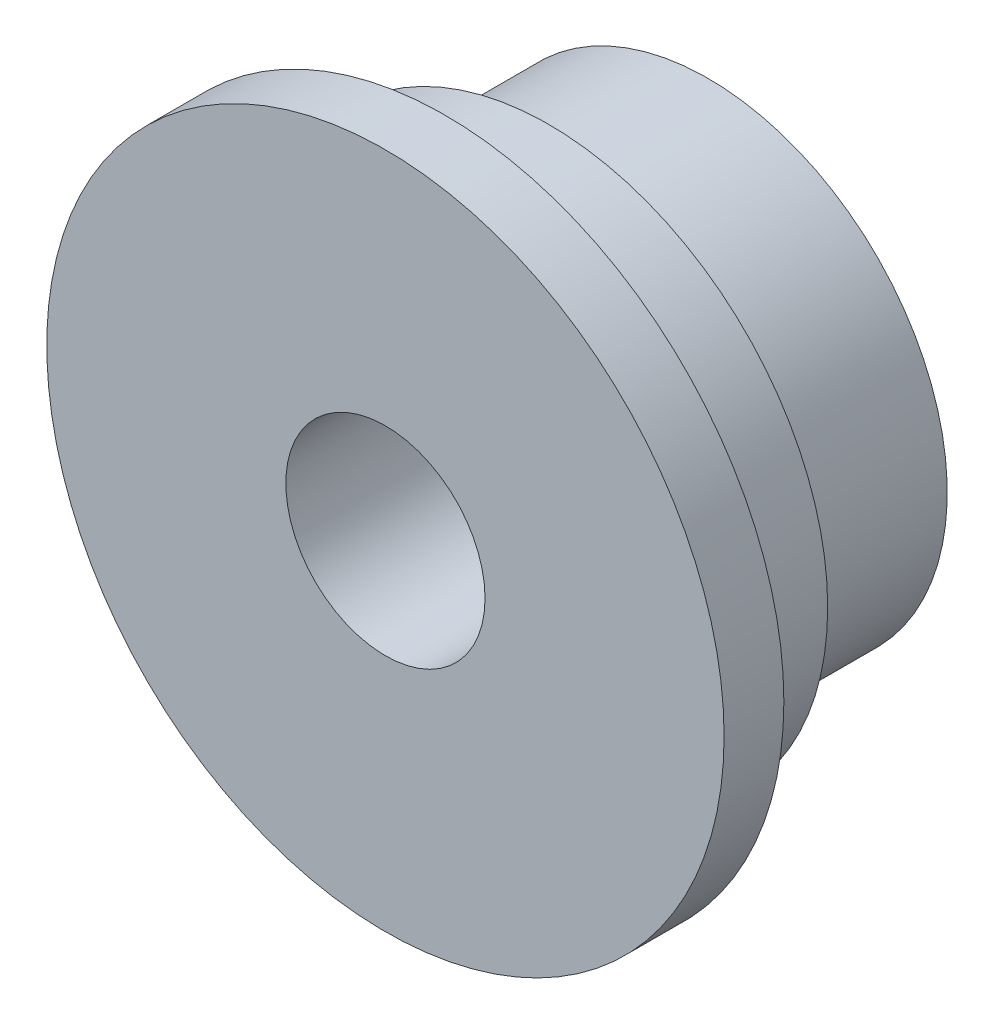
SolidWorks part; units mm, degrees
ref_plane "Front Plane" through (0, 0, 0) normal (0, 0, 1) x (1, 0, 0)
ref_plane "Top Plane" through (0, 0, 0) normal (0, 1, 0) x (1, 0, 0)
ref_plane "Right Plane" through (0, 0, 0) normal (1, 0, 0) x (0, 0, -1)
other "Configuration Table"
sketch "Sketch1" plane through (0, 0, 0) normal (0, 0, 1) x (1, 0, 0)
  circle A0 centre (0, 0) radius 70
  dimension "D1" = 140
extrude "Boss-Extrude1" add sketch "Sketch1" along normal up to surface (26 mm away)
sketch "Sketch2" plane through (0, 0, 26) normal (0, 0, 1) x (1, 0, 0)
  circle A0 centre (0, 0) radius 85
  dimension "D1" = 170
extrude "Boss-Extrude2" add sketch "Sketch2" along normal blind 15
sketch "Sketch3" plane through (0, 0, 0) normal (0, 0, -1) x (-1, 0, 0)
  circle A0 centre (0, 0) radius 60
  circle A1 centre (0, 0) radius 70 construction
  dimension "D1" = 10
extrude "Boss-Extrude3" add sketch "Sketch3" along normal blind 40
sketch "Sketch4" plane through (0, 0, 41) normal (0, 0, 1) x (1, 0, 0)
  circle A0 centre (0, 0) radius 25
  dimension "D1" = 50
extrude "Cut-Extrude1" cut sketch "Sketch4" against normal through all both and the other way through all
